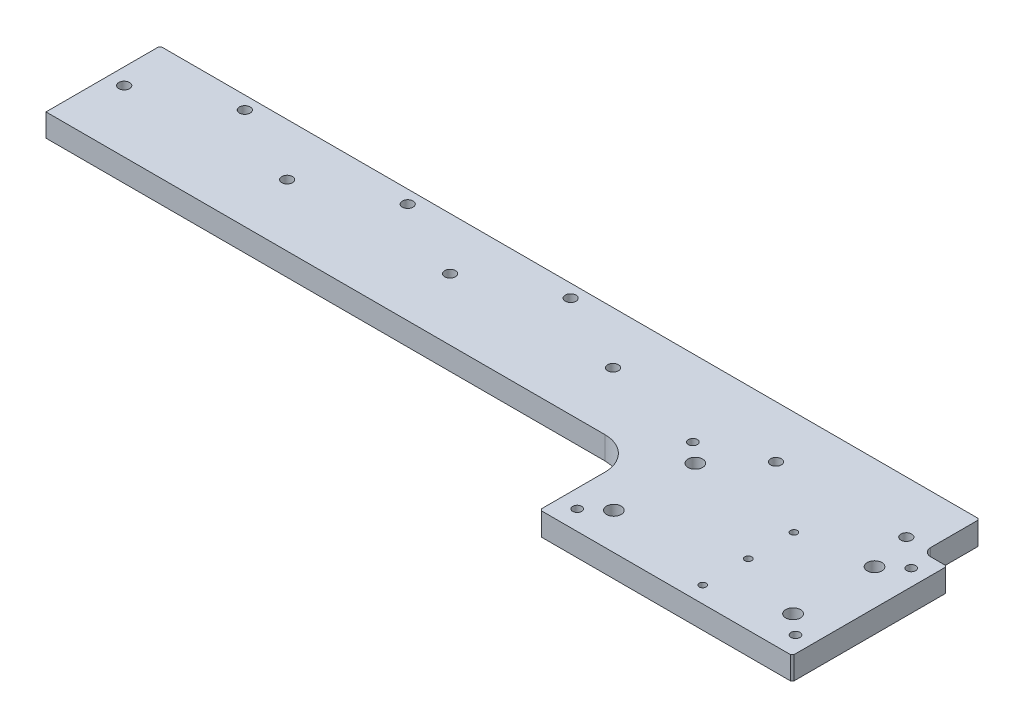
from build123d import *

# Parameters (mm, degrees)
SKETCH1_W                                            = 503
SKETCH1_H                                            = 130
BOSS_EXTRUDE1_DEPTH                                  = 7
SKETCH2_W                                            = 363
SKETCH2_H                                            = 60
CUT_EXTRUDE1_DEPTH                                   = 261.140827246
M5_TAPPED_HOLE1_D                                    = 4.2
HOLE_SIZE_PER_SOCKET_HEAD_CAP_SCREW_TYPE_D           = 6.6
HOLE_SIZE_PER_SOCKET_HEAD_CAP_SCREW_TYPE_CBORE_D     = 11
HOLE_SIZE_PER_SOCKET_HEAD_CAP_SCREW_TYPE_CBORE_DEPTH = 6.8
M8_CLEARANCE_HOLE1_D                                 = 9
HOLE_SIZE_PER_SOCKET_HEAD_CAP_SCREW_2_D              = 6.6
HOLE_SIZE_PER_SOCKET_HEAD_CAP_SCREW_2_CBORE_D        = 11
HOLE_SIZE_PER_SOCKET_HEAD_CAP_SCREW_2_CBORE_DEPTH    = 6.8
FILLET2_R                                            = 20
CHAMFER1_SIZE                                        = 1
SKETCH12_W                                           = 15
SKETCH12_H                                           = 95
BOSS_EXTRUDE2_DEPTH                                  = 14
SKETCH13_R                                           = 5
CUT_EXTRUDE2_DEPTH                                   = 10
M5_CLEARANCE_HOLE1_D                                 = 5.5
FILLET3_R                                            = 5
CHAMFER2_SIZE                                        = 1


with BuildPart() as part:
    # Sketch1 → Boss-Extrude1 (new, symmetric)
    with BuildSketch(Plane(origin=(0, 0, 0), x_dir=(1, 0, 0), z_dir=(0, 1, 0))):
        Rectangle(SKETCH1_W, SKETCH1_H)
    extrude(amount=BOSS_EXTRUDE1_DEPTH, both=True)

    # Sketch2 → Cut-Extrude1 (cut, through all)
    with BuildSketch(Plane(origin=(0, 7, 0), x_dir=(1, 0, 0), z_dir=(0, 1, 0))):
        with Locations((-70, -35)):
            Rectangle(SKETCH2_W, SKETCH2_H)
    extrude(amount=-CUT_EXTRUDE1_DEPTH, mode=Mode.SUBTRACT)

    # M5 Tapped Hole1 (through all)
    with Locations(Plane(origin=(0, 7, 0), x_dir=(1, 0, 0), z_dir=(0, 1, 0))):
        with Locations((201.5, -55), (201.5, -27), (201.5, 1)):
            Hole(M5_TAPPED_HOLE1_D / 2)

    # Hole Size per Socket Head Cap Screw Type (through all)
    with Locations(Plane(origin=(0, -7, 0), x_dir=(-1, 0, 0), z_dir=(0, -1, 0))):
        with Locations((-8.5, 57), (191.5, 57), (91.5, 57)):
            CounterBoreHole(HOLE_SIZE_PER_SOCKET_HEAD_CAP_SCREW_TYPE_D / 2, HOLE_SIZE_PER_SOCKET_HEAD_CAP_SCREW_TYPE_CBORE_D / 2, HOLE_SIZE_PER_SOCKET_HEAD_CAP_SCREW_TYPE_CBORE_DEPTH)

    # M8 Clearance Hole1 (through all)
    with Locations(Plane(origin=(0, 7, 0), x_dir=(1, 0, 0), z_dir=(0, 1, 0))):
        with Locations((134.5, 7.5), (244.5, -42.5), (134.5, -42.5), (244.5, 7.5)):
            Hole(M8_CLEARANCE_HOLE1_D / 2)

    # Hole Size per Socket Head Cap Screw  2 (through all)
    with Locations(Plane(origin=(0, -7, 0), x_dir=(-1, 0, 0), z_dir=(0, -1, 0))):
        with Locations((-238.5, 33), (241.5, 33), (141.5, 33), (41.5, 33), (-58.5, 33), (-158.5, 33)):
            CounterBoreHole(HOLE_SIZE_PER_SOCKET_HEAD_CAP_SCREW_2_D / 2, HOLE_SIZE_PER_SOCKET_HEAD_CAP_SCREW_2_CBORE_D / 2, HOLE_SIZE_PER_SOCKET_HEAD_CAP_SCREW_2_CBORE_DEPTH)

    # Fillet2
    fillet2_edges = [part.edges().sort_by_distance(p)[0] for p in [
        (111.5, 0, 5),
    ]]
    fillet(fillet2_edges, radius=FILLET2_R)

    # Chamfer1
    chamfer1_edges = [part.edges().sort_by_distance(p)[0] for p in [
        (111.5, 0, 65),
        (-251.5, 0, -65),
        (251.5, 0, -65),
    ]]
    chamfer(chamfer1_edges, length=CHAMFER1_SIZE)

    # Sketch12 → Boss-Extrude2 (add)
    with BuildSketch(Plane(origin=(0, 7, 0), x_dir=(1, 0, 0), z_dir=(0, 1, 0))):
        with Locations((259, -17.5)):
            Rectangle(SKETCH12_W, SKETCH12_H)
    extrude(amount=-BOSS_EXTRUDE2_DEPTH)

    # Sketch13 → Cut-Extrude2 (cut)
    with BuildSketch(Plane.XZ.offset(7)):
        with Locations(Location((122.5, 53, 0), (0, 0, 270))):
            Circle(SKETCH13_R)
        with Locations(Location((256.5, 53, 0), (0, 0, 90))):
            Circle(SKETCH13_R)
        with Locations(Location((256.5, -18, 0), (0, 0, 270))):
            Circle(SKETCH13_R)
        with Locations(Location((122.5, -18, 0), (0, 0, 90))):
            Circle(SKETCH13_R)
    extrude(amount=-CUT_EXTRUDE2_DEPTH, mode=Mode.SUBTRACT)

    # M5 Clearance Hole1 (through all)
    with Locations(Plane(origin=(0, 7, 0), x_dir=(1, 0, 0), z_dir=(0, 1, 0))):
        with Locations((122.5, 18), (122.5, -53), (256.5, -53), (256.5, 18)):
            Hole(M5_CLEARANCE_HOLE1_D / 2)

    # Fillet3
    fillet3_edges = [part.edges().sort_by_distance(p)[0] for p in [
        (251.5, 0, -30),
    ]]
    fillet(fillet3_edges, radius=FILLET3_R)

    # Chamfer2
    chamfer2_edges = [part.edges().sort_by_distance(p)[0] for p in [
        (266.5, 0, 65),
        (266.5, 0, -30),
    ]]
    chamfer(chamfer2_edges, length=CHAMFER2_SIZE)


solid = part.part
